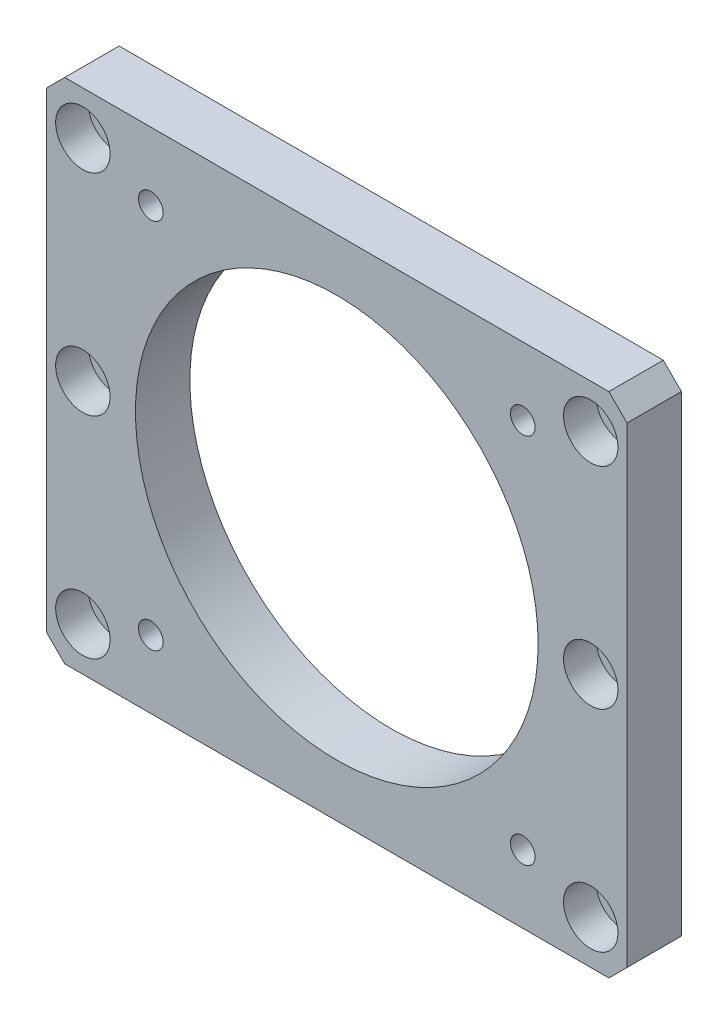
SolidWorks part; units mm, degrees
ref_plane "Front Plane" through (0, 0, 0) normal (0, 0, 1) x (1, 0, 0)
ref_plane "Top Plane" through (0, 0, 0) normal (0, 1, 0) x (1, 0, 0)
ref_plane "Right Plane" through (0, 0, 0) normal (1, 0, 0) x (0, 0, -1)
sketch "Sketch1" plane through (0, 0, 0) normal (0, 0, 1) x (1, 0, 0)
  line L0 (-80, 65) -> (-75, 70)
  line L1 (-75, -70) -> (75, -70)
  line L2 (-80, -65) -> (-80, 65)
  line L3 (-75, 70) -> (75, 70)
  line L4 (80, -65) -> (80, 65)
  line L5 (-80, -65) -> (-75, -70)
  line L6 (75, -70) -> (80, -65)
  line L7 (80, 65) -> (75, 70)
  circle A0 centre (0, 0) radius 55.5
  point P3 (-80, -70)
  point P4 (80, 70)
  point P5 (-80, 70)
  point P6 (80, -70)
  dimension "D5" = 111
  dimension "D1" = 140
  dimension "D2" = 160
  dimension "D3" = 70
  dimension "D4" = 80
extrude "Boss-Extrude1" add sketch "Sketch1" along normal blind 15
hole_wizard "M8 Tapped Hole1" positions "Sketch3" profile "Sketch2" tap size "M8" standard "GB"
sketch "Sketch3" plane through (0, 0, 15) normal (0, 0, 1) x (1, 0, 0)
  line L0 (0, 0) -> (51.2652, 51.2652) construction
  line L2 (0, 55.5) -> (0, -55.5) construction
  circle A0 centre (0, 0) radius 55.5 construction
  point P1 (51.2652, 51.2652)
  dimension "D1" = 45
  dimension "D2" = 72.5
sketch "Sketch2" plane through (51.2652, 51.2652, 15) normal (1, 0, 0) x (0, -1, 0)
  line L0 (0, 0) -> (0, 21.7929)
  line L1 (0, 21.7929) -> (3.4, 19.75)
  line L2 (3.4, 19.75) -> (3.4, 0)
  line L5 (3.4, 0) -> (0, 0)
  line L10 (0, 21.7929) -> (-3.4, 19.75) construction
  line L11 (0, -6.35) -> (0, 107.95) construction
  dimension "螺纹孔钻头直径" = 6.8
  dimension "螺纹孔钻头深度" = 19.75
  dimension "导头角度" = 118
cosmetic thread "Cosmetic Thread1" parameters "D1"=15, "D2"=8
pattern_circular "CirPattern1" count 4 over 360 about axis through (0, 0, 0) along (0, 0, 1) of "M8 Tapped Hole1"
hole_wizard "Hole size per socket head cap screw type1" positions "Sketch5" profile "Sketch4" counterbore size "M8" standard "Gb" end condition through all
sketch "Sketch5" plane through (37.8334, 52.116, 15) normal (0, 0, -1) x (-1, 0, 0)
  line L0 (-42.1666, -117.116) -> (-42.1666, 12.884) construction
  line L1 (37.8334, -52.116) -> (-59.9634, -52.116) construction
  point P1 (-32.1666, 5.884)
  point P19 (-32.1666, -52.116)
  point P35 (-32.1666, -110.116)
  dimension "D1" = 10
  dimension "D2" = 58
sketch "Sketch4" plane through (70, 58, 15) normal (1, 0, 0) x (0, -1, 0)
  line L0 (0, 0) -> (0, 15)
  line L1 (0, 15) -> (4.5, 15)
  line L3 (4.5, 15) -> (4.5, 9)
  line L4 (4.5, 9) -> (7.5, 9)
  line L5 (7.5, 9) -> (7.5, 0)
  line L7 (7.5, 0) -> (0, 0)
  line L11 (0, -6.35) -> (0, 107.95) construction
  dimension "通孔孔直径" = 9
  dimension "通孔孔深度" = 15
  dimension "柱形沉头孔直径" = 15
  dimension "柱形沉头孔深度" = 9
mirror "Mirror1" about plane through (0, 0, 0) normal (1, 0, 0) of "Hole size per socket head cap screw type1"
